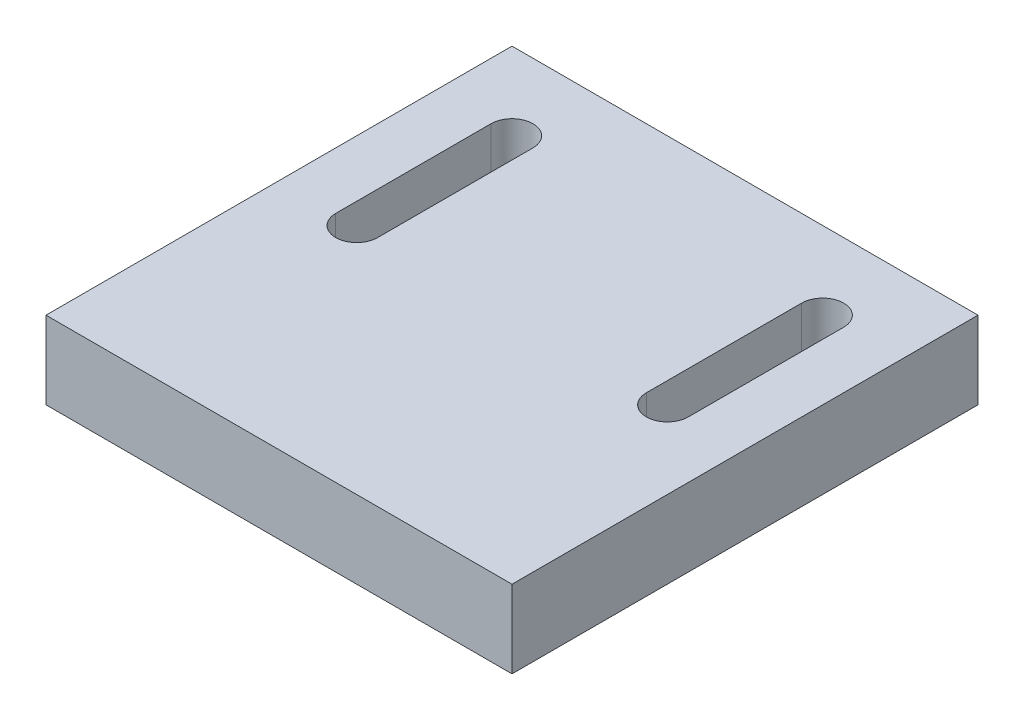
from build123d import *

# Parameters (mm, degrees)
SKETCH1_W           = 60
SKETCH1_H           = 60
BOSS_EXTRUDE1_DEPTH = 10
CUT_EXTRUDE1_DEPTH  = 44.588989435


with BuildPart() as part:
    # Sketch1 → Boss-Extrude1 (new body)
    with BuildSketch(Plane(origin=(0, 0, 0), x_dir=(1, 0, 0), z_dir=(0, 1, 0))):
        Rectangle(SKETCH1_W, SKETCH1_H)
    extrude(amount=BOSS_EXTRUDE1_DEPTH)

    # Sketch2 → Cut-Extrude1 (cut, through all)
    with BuildSketch(Plane(origin=(0, 10, 0), x_dir=(1, 0, 0), z_dir=(0, 1, 0))):
        with BuildLine():
            Line((17.3, 0), (17.3, 20))
            ThreePointArc((17.3, 20), (20, 22.7), (22.7, 20))
            Line((22.7, 20), (22.7, 0))
            ThreePointArc((22.7, 0), (20, -2.7), (17.3, 0))
        make_face()
    cut_extrude1 = extrude(amount=-CUT_EXTRUDE1_DEPTH, mode=Mode.SUBTRACT)

    # Mirror1: Cut-Extrude1 across plane
    add(cut_extrude1.mirror(Plane(origin=(0, 0, 0), x_dir=(0, 0, 1), z_dir=(1, 0, 0))), mode=Mode.SUBTRACT)


solid = part.part
